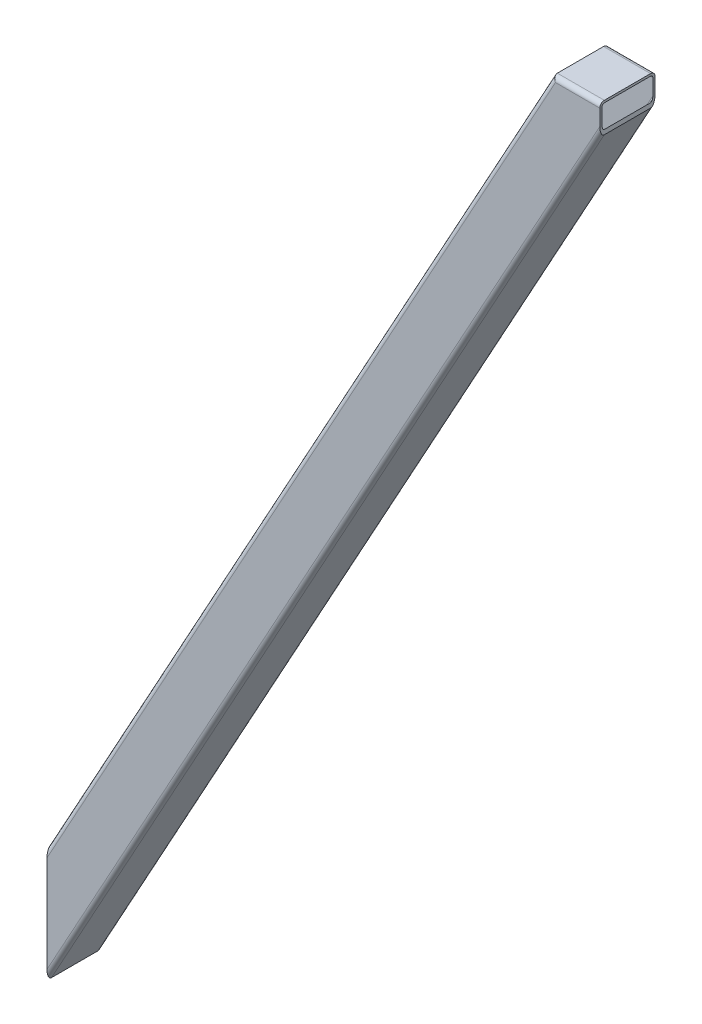
from build123d import *

# Parameters (mm, degrees)
BOSS_EXTRUDE1_DEPTH   = 100
SHELL1_T              = -4
FILLET1_R             = 8.2
FILLET2_R             = 4.2
M8_TAPPED_HOLE1_D     = 6.8
M8_TAPPED_HOLE1_DEPTH = 19.75
M8_TAPPED_HOLE1_TIP   = 2.042926105


with BuildPart() as part:
    # Sketch1 → Boss-Extrude1 (new body)
    with BuildSketch(Plane.XY):
        Polygon((0, 0), (0, 208.736831721), (915, 1874.433314365), (1000, 1874.433314365), (1000, 1820.433314365), align=None)
    extrude(amount=BOSS_EXTRUDE1_DEPTH)

    # Shell1
    shell1_openings = [part.faces().sort_by_distance(p)[0] for p in [
        (0, 104.36841586, 50),
        (1000, 1847.433314365, 50),
    ]]
    offset(amount=SHELL1_T, openings=shell1_openings, kind=Kind.INTERSECTION)

    # Fillet1
    fillet1_edges = [part.edges().sort_by_distance(p)[0] for p in [
        (457.5, 1041.585073043, 100),
        (957.5, 1874.433314365, 100),
        (957.5, 1874.433314365, 0),
        (457.5, 1041.585073043, 0),
        (500, 910.216657182, 0),
        (500, 910.216657182, 100),
    ]]
    fillet(fillet1_edges, radius=FILLET1_R)

    # Fillet2
    fillet2_edges = [part.edges().sort_by_distance(p)[0] for p in [
        (958.683247588, 1870.433314365, 96),
        (458.683247588, 1035.431049715, 96),
        (500, 918.524703838, 96),
        (500, 918.524703838, 4),
        (458.683247588, 1035.431049715, 4),
        (958.683247588, 1870.433314365, 4),
    ]]
    fillet(fillet2_edges, radius=FILLET2_R)

    # M8 Tapped Hole1
    with Locations(Plane(origin=(0, 0, 0), x_dir=(-1, 0, 0), z_dir=(0, 0, -1))):
        with Locations((-316, 708.43)):
            Hole(M8_TAPPED_HOLE1_D / 2, depth=M8_TAPPED_HOLE1_DEPTH)
            with Locations((0, 0, -(M8_TAPPED_HOLE1_DEPTH + M8_TAPPED_HOLE1_TIP / 2))):  # 118° drill point
                Cone(0, M8_TAPPED_HOLE1_D / 2, M8_TAPPED_HOLE1_TIP, mode=Mode.SUBTRACT)


solid = part.part
